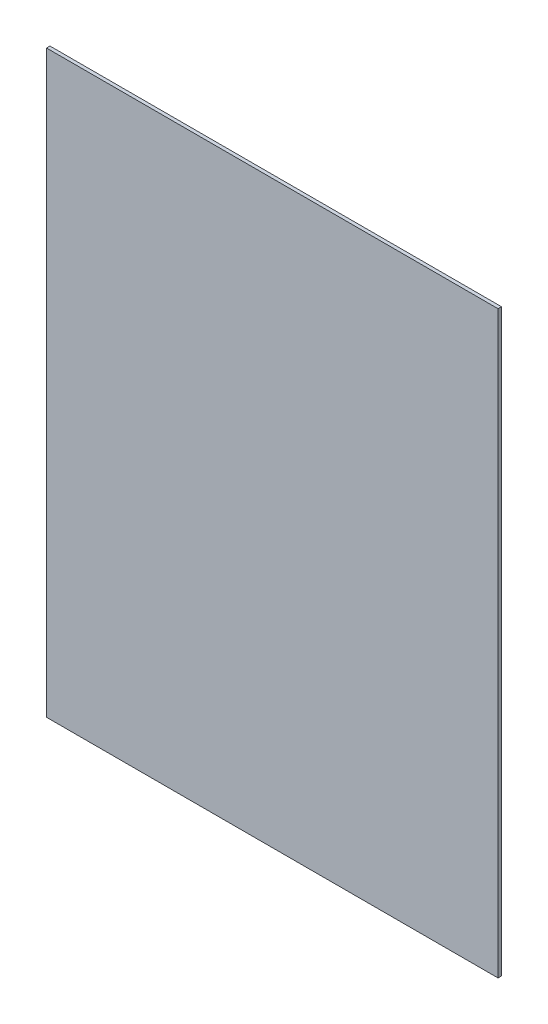
from build123d import *

# Parameters (mm, degrees)
SKETCH_1_W      = 656
SKETCH_1_H      = 842
EXTRUDE_1_DEPTH = 5


with BuildPart() as part:
    # 草图1 → 凸台-拉伸1 (new body)
    with BuildSketch(Plane.XY):
        Rectangle(SKETCH_1_W, SKETCH_1_H)
    extrude(amount=EXTRUDE_1_DEPTH)


solid = part.part
